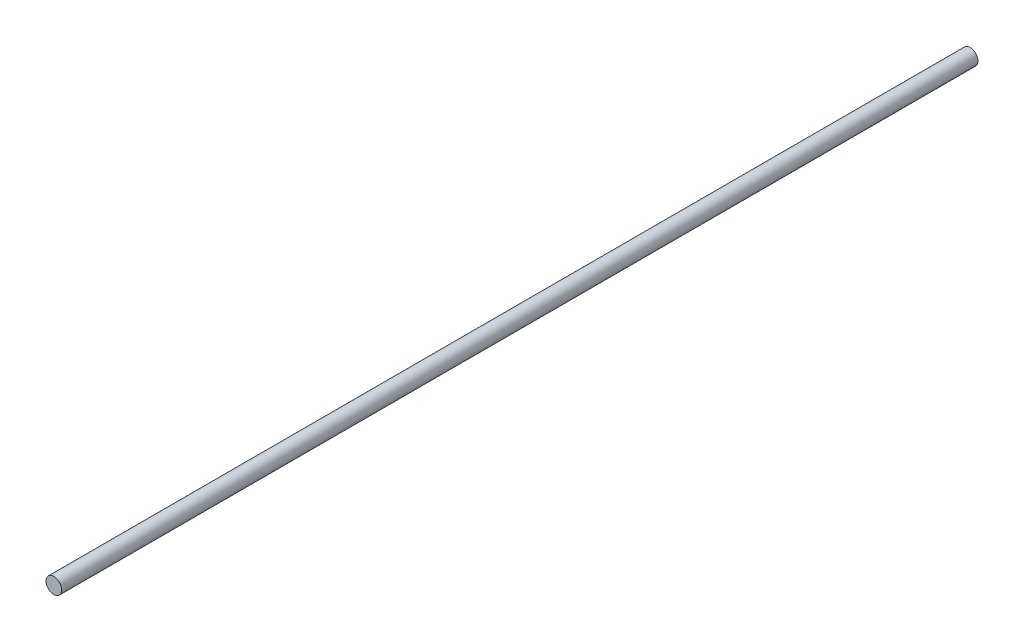
from build123d import *

# Parameters (mm, degrees)
SKETCH1_R           = 3
BOSS_EXTRUDE1_DEPTH = 350


with BuildPart() as part:
    # Sketch1 → Boss-Extrude1 (new body)
    with BuildSketch(Plane.XY):
        Circle(SKETCH1_R)
    extrude(amount=BOSS_EXTRUDE1_DEPTH)


solid = part.part
